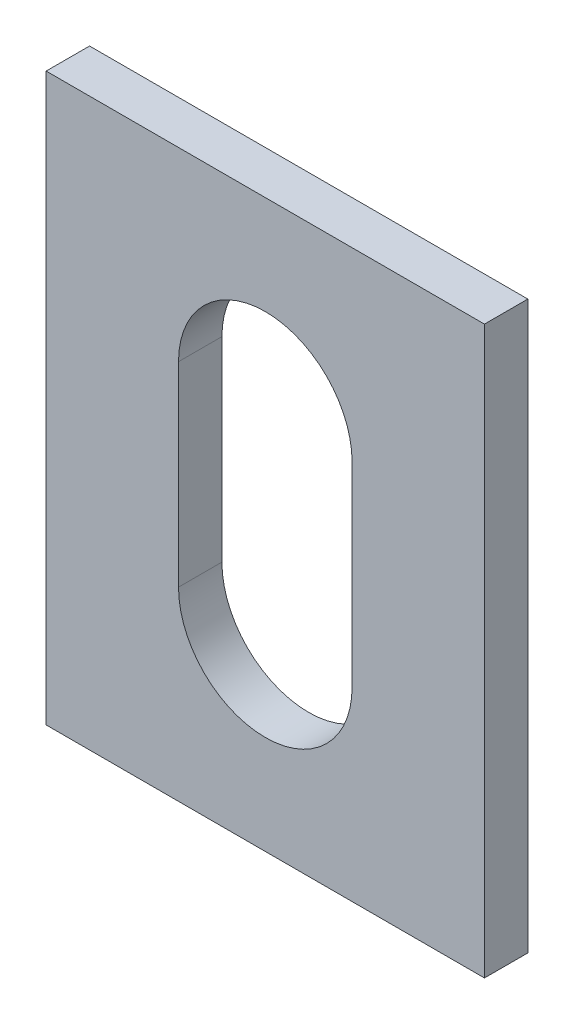
SolidWorks part; units mm, degrees
material "Q345 "
ref_plane "前视基准面" through (0, 0, 0) normal (0, 0, 1) x (1, 0, 0)
ref_plane "上视基准面" through (0, 0, 0) normal (0, 1, 0) x (1, 0, 0)
ref_plane "右视基准面" through (0, 0, 0) normal (1, 0, 0) x (0, 0, -1)
sketch "草图1" plane through (0, 0, 0) normal (0, 0, 1) x (1, 0, 0)
  line L0 (-75, 3.9199) -> (-75, -36.96) construction
  line L1 (-75, 5) -> (-277, 5)
  line L2 (-75, 5) -> (-75, -256)
  line L3 (-75, -256) -> (-277, -256)
  line L4 (-277, 5) -> (-277, -256)
  line L5 (-277, -254.9199) -> (-277, -214.04) construction
  line L6 (-277, -261) -> (-75, -261) construction
  line L7 (-75, 10) -> (-277, 10) construction
  dimension "D1" = 5
  dimension "D2" = 5
extrude "凸台-拉伸1" add sketch "草图1" along normal blind 20
sketch "草图2" plane through (0, 0, 20) normal (0, 0, 1) x (1, 0, 0)
  line L0 (-176, -256) -> (-176, 5) construction
  line L1 (-277, -256) -> (-75, -256) construction
  line L2 (-75, 5) -> (-277, 5) construction
  line L3 (-176, -170.5) -> (-176, -80.5) construction
  line L4 (-216, -170.5) -> (-216, -80.5)
  line L5 (-136, -170.5) -> (-136, -80.5)
  arc A0 (-216, -170.5) -> (-136, -170.5) centre (-176, -170.5) ccw
  arc A1 (-136, -80.5) -> (-216, -80.5) centre (-176, -80.5) ccw
  point P8 (-176, -125.5)
  dimension "D1" = 40
  dimension "D2" = 90
extrude "切除-拉伸1" cut sketch "草图2" against normal through all
